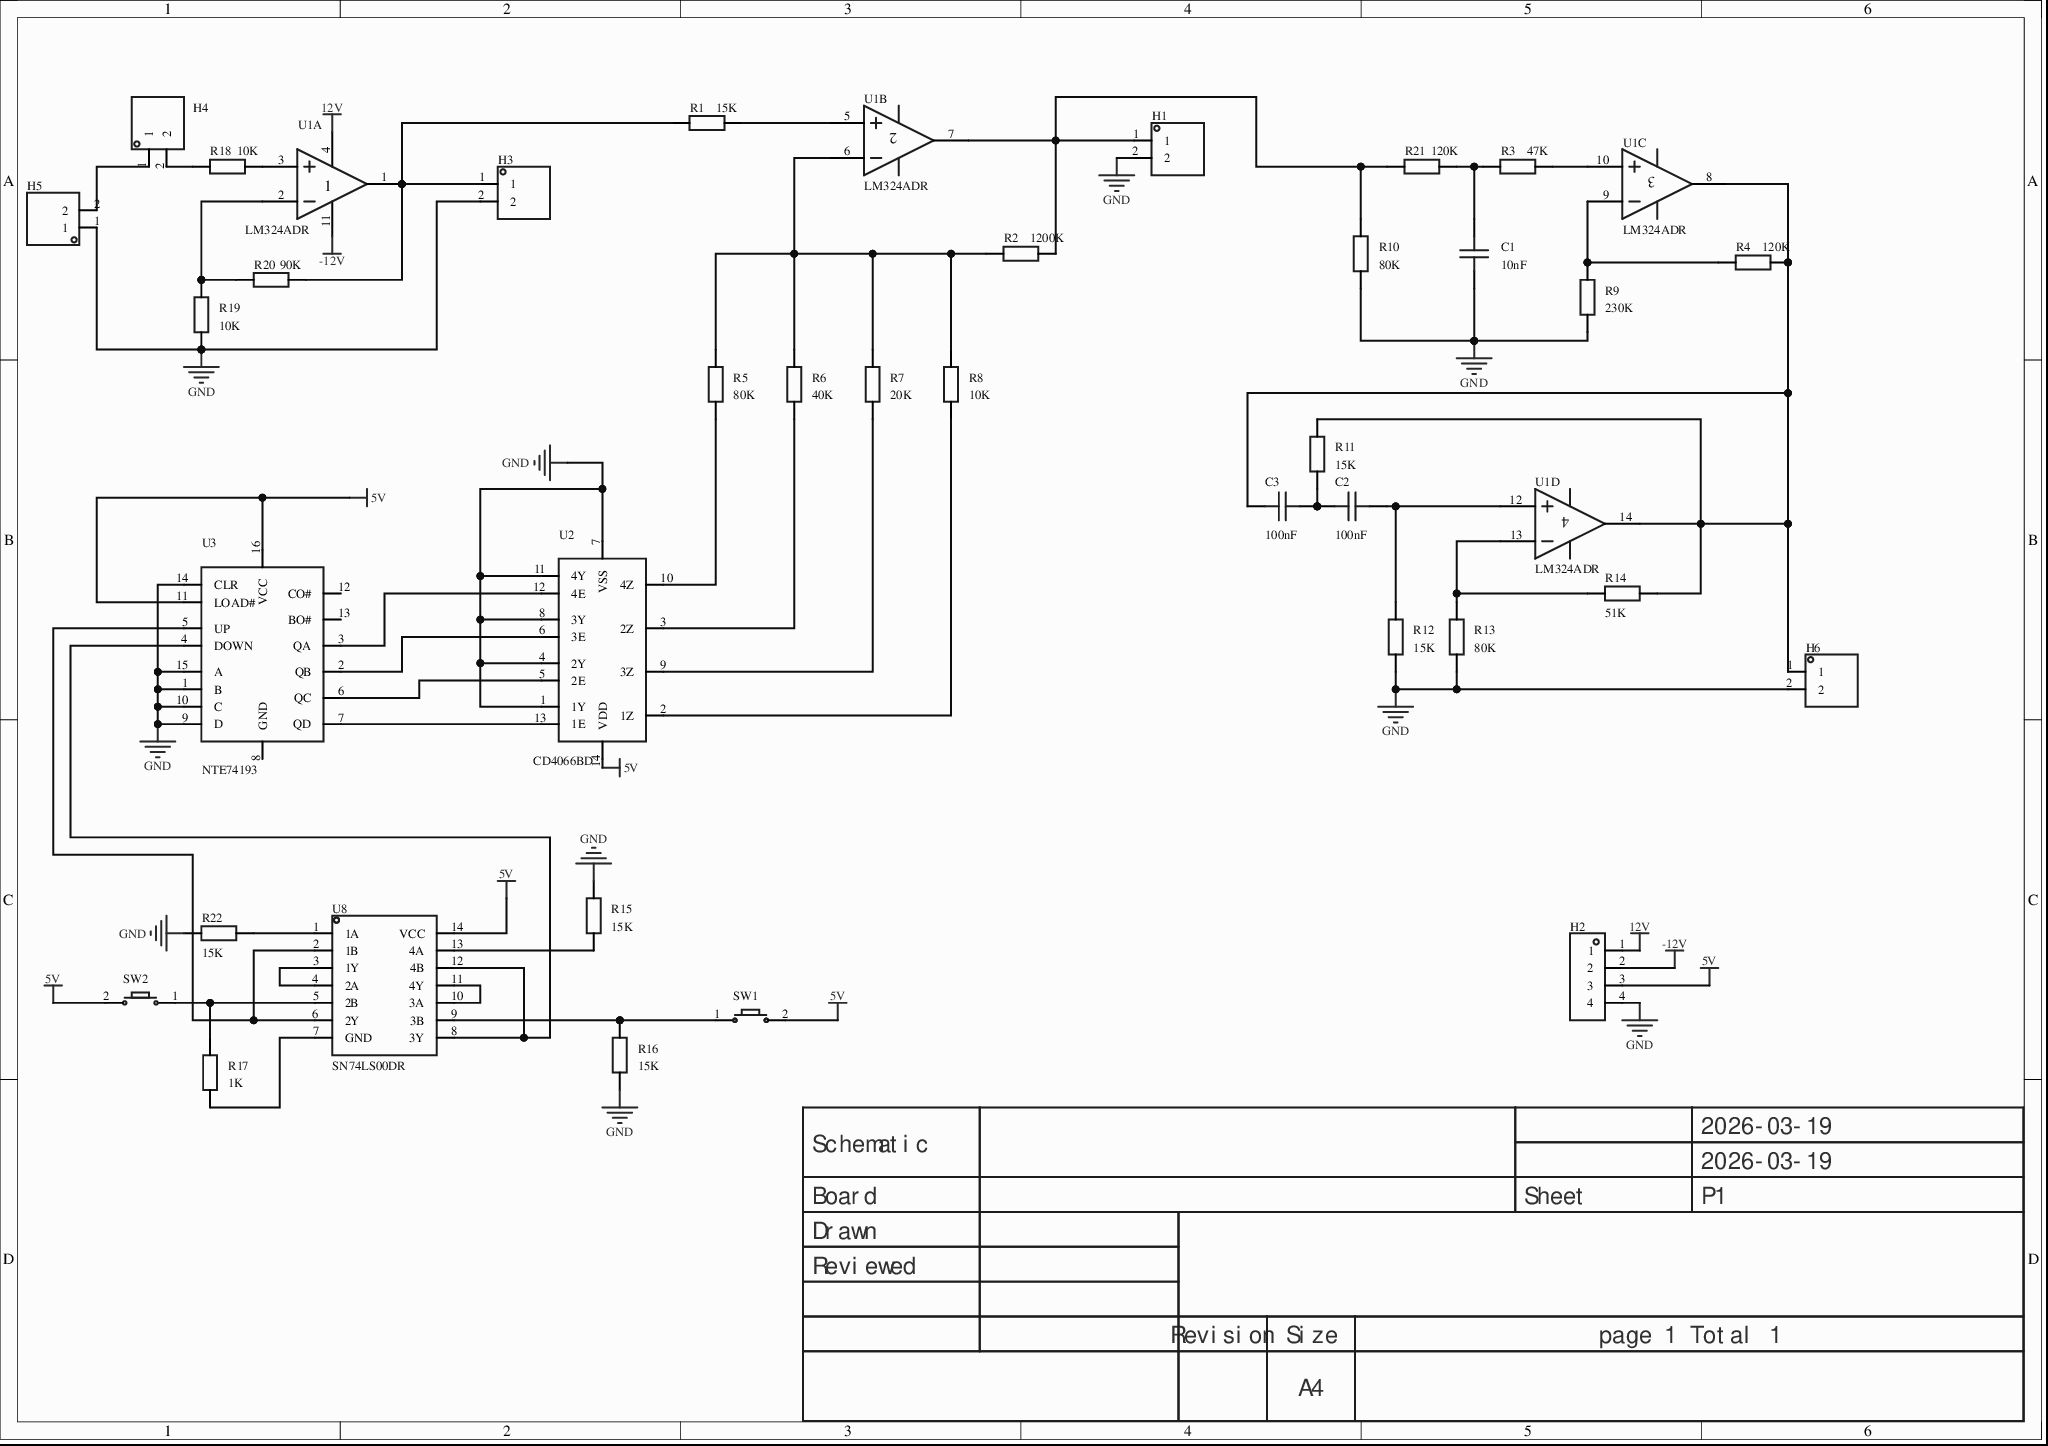
[diagram p0: MISC51958-3.schdoc]
# Altium project MISC51958-2.PrjPcb
1 sheet, 37 parts. Net scope: global (net labels, ports and power ports of the same name join across sheets).
Board file: MISC51958.pcbdoc

## Sheet MISC51958-3.schdoc
size 297 x 209 mm; Version: V1.0; @Project Name: MISC51958; @Update Date: 2026-03-19; @Create Date: 2026-03-19; @Board Name: MISC51958; @Create Time: 16:23:48; @Page Count: 1; @Page No: 1; @Schematic Name: MISC51958; @Update Time: 16:23:48; Size: A4

### Parts
C1  10nF  [CAP-TH_L5.0-W2.5-P5.00-D1.0]
C2  100nF  [CAP-TH_L5.0-W2.5-P5.00-D1.0]
C3  100nF  [CAP-TH_L5.0-W2.5-P5.00-D1.0]
H1  (no value)  [HDR-TH_2P-P2.54-V-M-1]
H2  (no value)  [HDR-TH_4P-P2.54-V-M]
H3  (no value)  [HDR-TH_2P-P2.54-V-M-1]
H4  (no value)  [HDR-TH_2P-P2.54-V-M-1]
H5  (no value)  [HDR-TH_2P-P2.54-V-M-1]
H6  (no value)  [HDR-TH_2P-P2.54-V-M-1]
R1  15K  [Res_1/8W]
R2  1200K  [Res_1/8W]
R3  47K  [Res_1/8W]
R4  120K  [Res_1/8W]
R5  80K  [Res_1/8W]
R6  40K  [Res_1/8W]
R7  20K  [Res_1/8W]
R8  10K  [Res_1/8W]
R9  230K  [Res_1/8W]
R10  80K  [Res_1/8W]
R11  15K  [Res_1/8W]
R12  15K  [Res_1/8W]
R13  80K  [Res_1/8W]
R14  51K  [Res_1/8W]
R15  15K  [Res_1/8W]
R16  15K  [Res_1/8W]
R17  1K  [Res_1/8W]
R18  10K  [Res_1/8W]
R19  10K  [Res_1/8W]
R20  90K  [Res_1/8W]
R21  120K  [Res_1/8W]
R22  15K  [Res_1/8W]
SW1  (no value)  [Key_SMD_3x4x2]
SW2  (no value)  [Key_SMD_3x4x2]
U1  LM324ADR  [SOP-14_L8.6-W3.9-P1.27-LS6.0-BL]  (parts A,B,C,D of 4)
U2  CD4066BD  [SOP-14_L8.6-W3.9-P1.27-LS6.0-BL]
U3  NTE74193  [PDIP-16_L19.7-W6.6-P2.54-LS7.6-BL]
U8  SN74LS00DR  [SOIC-14_L8.7-W3.9-P1.27-LS6.0-BL]

### Nets
5V: H2.3 SW1.2 SW2.2 U2.14(VDD) U3.11(LOAD#) U3.16(VCC) U8.14(VCC)
12V: H2.1 U1.4(VCC)
-12V: H2.2 U1.11(GND)
GND: C1.1 H1.2 H2.4 H3.2 H5.1 H6.2 R9.1 R10.1 R12.1 R13.1 R15.2 R16.1 R19.1 R22.2 U2.1(1Y) U2.4(2Y) U2.7(VSS) U2.8(3Y) U2.11(4Y) U3.1(B) U3.9(D) U3.10(C) U3.14(CLR) U3.15(A)
NetC1_2: C1.2 R3.1 R21.2
NetC2_1: C2.1 R12.2 U1.12(4IN+)
NetC2_2: C2.2 C3.1 R11.1
NetC3_2: C3.2 H6.1 R4.2 R11.2 R14.1 U1.8(3OUT) U1.14(4OUT)
NetH1_1: H1.1 R2.2 R10.2 R21.1 U1.7(2OUT)
NetH3_1: H3.1 R1.1 R20.2 U1.1(1OUT)
NetH4_1: H4.1 H5.2
NetH4_2: H4.2 R18.1
NetR1_2: R1.2 U1.5(2IN+)
NetR2_1: R2.1 R5.2 R6.2 R7.2 R8.2 U1.6(2IN-)
NetR3_2: R3.2 U1.10(3IN+)
NetR4_1: R4.1 R9.2 U1.9(3IN-)
NetR5_1: R5.1 U2.10(4Z)
NetR6_1: R6.1 U2.3(2Z)
NetR7_1: R7.1 U2.9(3Z)
NetR8_1: R8.1 U2.2(1Z)
NetR13_2: R13.2 R14.2 U1.13(4IN-)
NetR15_1: R15.1 U8.13(4A)
NetR16_2: R16.2 SW1.1 U8.9(3B)
NetR17_1: R17.1 U8.7(GND)
NetR17_2: R17.2 SW2.1 U8.5(2B)
NetR18_2: R18.2 U1.3(1IN-)
NetR19_2: R19.2 R20.1 U1.2(1IN+)
NetR22_1: R22.1 U8.1(1A)
NetU2_5: U2.5(2E) U3.6(QC)
NetU2_6: U2.6(3E) U3.2(QB)
NetU2_12: U2.12(4E) U3.3(QA)
NetU2_13: U2.13(1E) U3.7(QD)
NetU3_4: U3.4(DOWN) U8.8(3Y) U8.12(4B)
NetU3_5: U3.5(UP) U8.2(1B) U8.6(2Y)
NetU8_3: U8.3(1Y) U8.4(2A)
NetU8_10: U8.10(3A) U8.11(4Y)

Not connected (* = marked no-connect by the designer): U3 8(GND) 12(CO#) 13(BO#)

### Notes on the sheet
- 2026-03-19
- Schematic
- Board
- Sheet
- P1
- Drawn
- Reviewed
- Revision
- Size
- A4
- page 1 Total 1

### Library data of the parts
C1-C3 = CAP_0603: Symbol: Capacitance; 3D Model: ac125912035d415993ca9572d50418b10819f05c4eef4c71ace90d822a990e87; 3D Model Transform: 62.992,31.496,0,0,0,0,0,0,0; ConvertToPcb: yes; ModelName: C0603_L1.6-W0.8-H0.8; Device: CAP_0603; Supplier Footprint: 0603; AddInBom: yes; FootprintName: CAP-TH_L5.0-W2.5-P5.00-D1.0
  C1: Value: 10nF
  C2 C3: Value: 100nF
H1 H3-H6 = HDR-M_2.54_1x2P: Symbol: 210S-1*2P L=11.6MMGold-plated black; 3D Model: 79b2e9f2d70a4d68a1b7098f27c6d4c50819f05c4eef4c71ace90d822a990e87; 3D Model Transform: 200,100,0,0,0,0,0,0,-118.11; ConvertToPcb: yes; ModelName: HDR-M-2.54_1x2; Device: HDR-M_2.54_1x2P; Supplier Part: C124375; Supplier Footprint: 插件; AddInBom: yes; FootprintName: HDR-TH_2P-P2.54-V-M-1
H2 = HDR-M_2.54_1x4P: Symbol: PZ254V-11-04P; ConvertToPcb: yes; ModelId: 112f4d05e8d64e99ab9a333894bea4f90819f05c4eef4c71ace90d822a990e87; ModelName: HDR-TH_4P-P2.54-M-LI-1X4P; ModelTransform: 399.999,104.7242,0,0,0,0,0,0,-118.11; Device: HDR-M_2.54_1x4P; AddInBom: yes; SupplierPart: C492403; Supplier Footprint: 插件; FootprintName: HDR-TH_4P-P2.54-V-M
R1-R22 = Res_0603: Symbol: Resistor; 3D Model: fc143cca1e79419f9cd78b61e9279f080819f05c4eef4c71ace90d822a990e87; 3D Model Transform: 31.8897,63.7794,0,90,0,0,0,0,0; ConvertToPcb: yes; ModelName: R0603; Device: Res_0603; Supplier Footprint: 0603; AddInBom: yes; FootprintName: Res_1/8W
  R1 R11 R12 R15 R16 R22: Value: 15K
  R2: Value: 1200K
  R3: Value: 47K
  R4 R21: Value: 120K
  R5 R10 R13: Value: 80K
  R6: Value: 40K
  R7: Value: 20K
  R8 R18 R19: Value: 10K
  R9: Value: 230K
  R14: Value: 51K
  R17: Value: 1K
  R20: Value: 90K
SW1 SW2 = Key_SMD_3x4x2: Symbol: Tact switch x2; ConvertToPcb: yes; ModelId: 63599cce708d48afbce1b0db003544770819f05c4eef4c71ace90d822a990e87; ModelName: SW-SMD_L4.0-W2.9-H2-LS5.0; ModelTransform: 196.85,114.17,79.13,0,0,0,0,0,0; Device: Key_SMD_3x4x2; AddInBom: yes; Supplier Footprint: SMD; FootprintName: Key_SMD_3x4x2
U1 = LM324ADR_C2837469: Amplifiers: quad; rail-to-rail: -; GBP: -; input offset voltage (Vos): 9mV; input bias current (Ib): 250nA;; Manufacturer: UMW(友台半导体); Relevance: []; 3D Model: 520b569c4a2341089bdfdd9bf52b86190819f05c4eef4c71ace90d822a990e87; 3D Model Transform: 339.763,236.22,0,0,0,0,0,0,0; Input Offset Voltage Drift(Vos TC): 7uV/℃; Common Mode Rejection Ratio(CMRR): 80dB; AddInBom: yes; Symbol: LM324ADR_C2837469; Device: LM324ADR_C2837469; LCSC Part Name: LM324ADR; Supplier Part: C2837469; Manufacturer Part: LM324ADR; Supplier Footprint: SOP-14; JLCPCB Part Class: Extended Part; Datasheet: https://example.com/datasheet/LM324ADR/3008835.html; Supplier: LCSC; Number of Channels: Quad; Rail to Rail: -; Gain Bandwidth Product: -; Vos - Input Offset Voltage: 9mV; Ib - Input Bias Current: 250nA; Input Offset Current(Ios): -; Input offset current drift(Ios TC): -; Quiescent Current: -; Output Current: -; Operating Temperature: -40℃~+85℃; ConvertToPcb: yes; FootprintName: SOP-14_L8.6-W3.9-P1.27-LS6.0-BL; ModelName: SOP-14_L8.6-W3.9-P1.27-LS6.0-BL
U2 = CD4066BD: Switch circuit: -; on-resistance (Ron): 1.05kΩ;; Manufacturer: HTC; 3D Model: 520b569c4a2341089bdfdd9bf52b86190819f05c4eef4c71ace90d822a990e87; 3D Model Transform: 339.763,236.22,0,0,0,0,0,0,0; Voltage - Supply: 3V~18V; Con: 7.5pF; Bandwidth: 40MHz; Propagation Delay (tpd): 40ns; AddInBom: yes; Symbol: CD4066BD; Device: CD4066BD; LCSC Part Name: CD4066BD; Supplier Part: C558790; Manufacturer Part: CD4066BD; Supplier Footprint: SOP-14; JLCPCB Part Class: Extended Part; Datasheet: https://example.com/datasheet/CD4066BD/582253.html; Supplier: LCSC; Switch Circuit: -; Ron: 1.05kΩ; Operating Temperature: -55℃~+125℃; ConvertToPcb: yes; FootprintName: SOP-14_L8.6-W3.9-P1.27-LS6.0-BL; ModelName: SOP-14_L8.6-W3.9-P1.27-LS6.0-BL
U3 = NTE74193: Operating voltage: -; component count: 1; count rate: 32MHz;; Manufacturer: NTE ELECTRONICS, INC.; 3D Model: 60304d8eb9b246fdb135cb3d16f241a80819f05c4eef4c71ace90d822a990e87; 3D Model Transform: 787.4,311.8104,0,0,0,0,0,0,-118.11; Logic Type: Divide by 2; Direction: Down counter; up counter; Number of Elements: 1; Reset: Asynchronous; Timing: Synchronous; AddInBom: yes; ModelName: PDIP-16_L19.7-W6.6-H5.1-P2.54-LS7.6-BL; Symbol: NTE74193; Device: NTE74193; LCSC Part Name: NTE74193; Supplier Part: C6345915; Manufacturer Part: NTE74193; Supplier Footprint: PDIP-16; JLCPCB Part Class: Extended Part; Datasheet: https://example.com/pdf/source/20240116/CF6500B458CC39AD140C0B858B31AFAA.pdf; Supplier: LCSC; Voltage - Supply: -; Count Rate: 32MHz; Operating Temperature: 0℃~+70℃; ConvertToPcb: yes; FootprintName: PDIP-16_L19.7-W6.6-P2.54-LS7.6-BL
U8 = SN74LS00DR: Logic type: NAND gate; channels: 4; operating voltage: 4.75V~5.25V; propagation delay (tpd): 15ns@5V,15pF;; Manufacturer: TI(德州仪器); AddInBom: yes; ModelId: 8dbf5b715d42428c85558507ae5a252b0819f05c4eef4c71ace90d822a990e87; ModelName: SOIC-14_L8.6-W3.9-H1.8-LS6.0-P1.27; ModelTransform: 338.583,236.22,0,0,0,0,0,0.001,0; Number of Channels: 4; Current - Output Low(IOL): 8mA; Current - Output High(IOH): 400uA; Input Logic Level - High: 2V; Input Logic Level - Low: 800mV; Output Logic Level - High: 2.5V; Output Logic Level - Low: 500mV; Input Number: 2; Symbol: SN74LS00DR; Device: SN74LS00DR; LCSC Part Name: 四路 2 输入正与非门; SupplierPart: C74558; ManufacturerPart: SN74LS00DR; Supplier Footprint: SOIC-14; JLCPCB Part Class: Extended Part; Supplier: LCSC; ConvertToPcb: yes; FootprintName: SOIC-14_L8.7-W3.9-P1.27-LS6.0-BL; Logic Type: NAND gate; Voltage - Supply: 4.75V~5.25V; Series: 74LS series; Propagation Delay: 15ns@5V,15pF; Operating Temperature: 0℃~+70℃